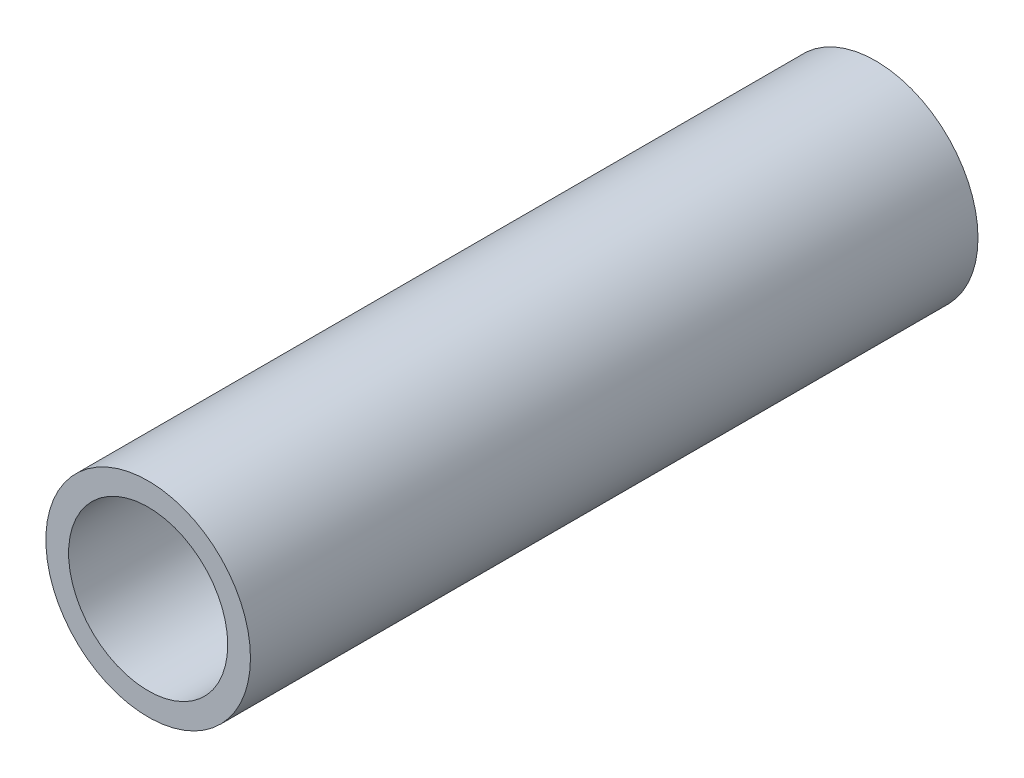
SolidWorks part; units mm, degrees
material "45"
ref_plane "Front Plane" through (0, 0, 0) normal (0, 0, 1) x (1, 0, 0)
ref_plane "Top Plane" through (0, 0, 0) normal (0, 1, 0) x (1, 0, 0)
ref_plane "Right Plane" through (0, 0, 0) normal (1, 0, 0) x (0, 0, -1)
sketch "Sketch1" plane through (0, 0, 0) normal (0, 0, 1) x (1, 0, 0)
  circle A0 centre (0, 0) radius 4.5
  circle A1 centre (0, 0) radius 3.5
  dimension "D1" = 7
  dimension "D2" = 9
extrude "Boss-Extrude1" add sketch "Sketch1" along normal blind 32
